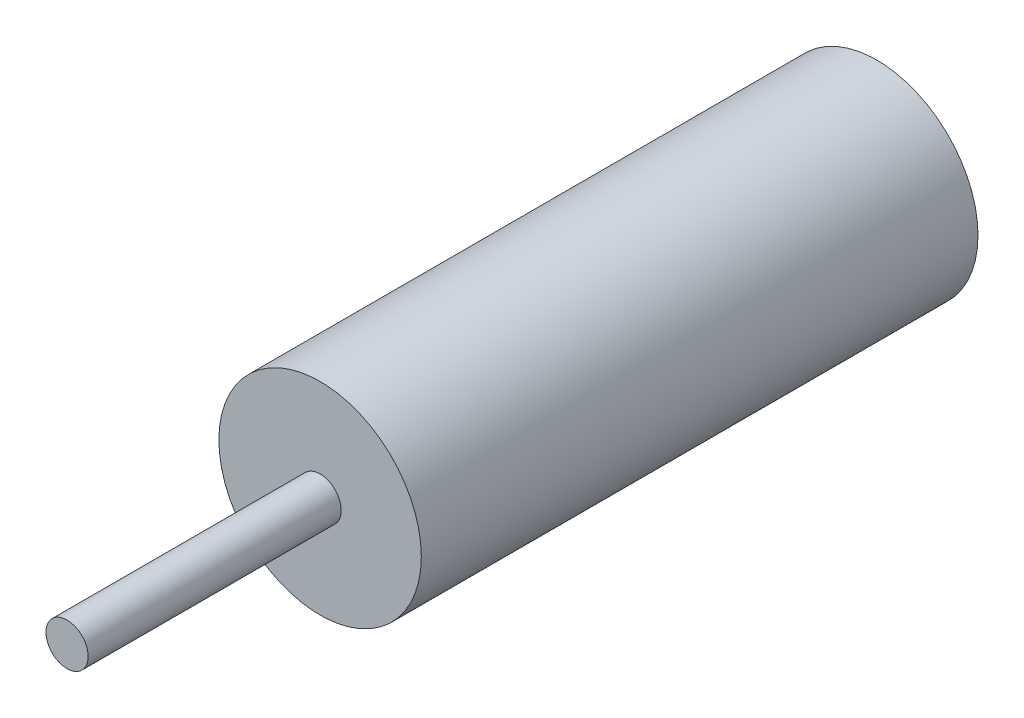
SolidWorks part; units mm, degrees
ref_plane "前视基准面" through (0, 0, 0) normal (0, 0, 1) x (1, 0, 0)
ref_plane "上视基准面" through (0, 0, 0) normal (0, 1, 0) x (1, 0, 0)
ref_plane "右视基准面" through (0, 0, 0) normal (1, 0, 0) x (0, 0, -1)
sketch "草图1" plane through (0, 0, 0) normal (0, 0, 1) x (1, 0, 0)
  circle A0 centre (0, 0) radius 6
  dimension "D1" = 12
extrude "凸台-拉伸1" add sketch "草图1" along normal blind 33
cosmetic thread "装饰螺纹线1" parameters "D2"=11
sketch "草图2" plane through (0, 0, 33) normal (0, 0, 1) x (1, 0, 0)
  circle A0 centre (0, 0) radius 1.25
  dimension "D1" = 2.5
extrude "凸台-拉伸2" add sketch "草图2" along normal blind 15
